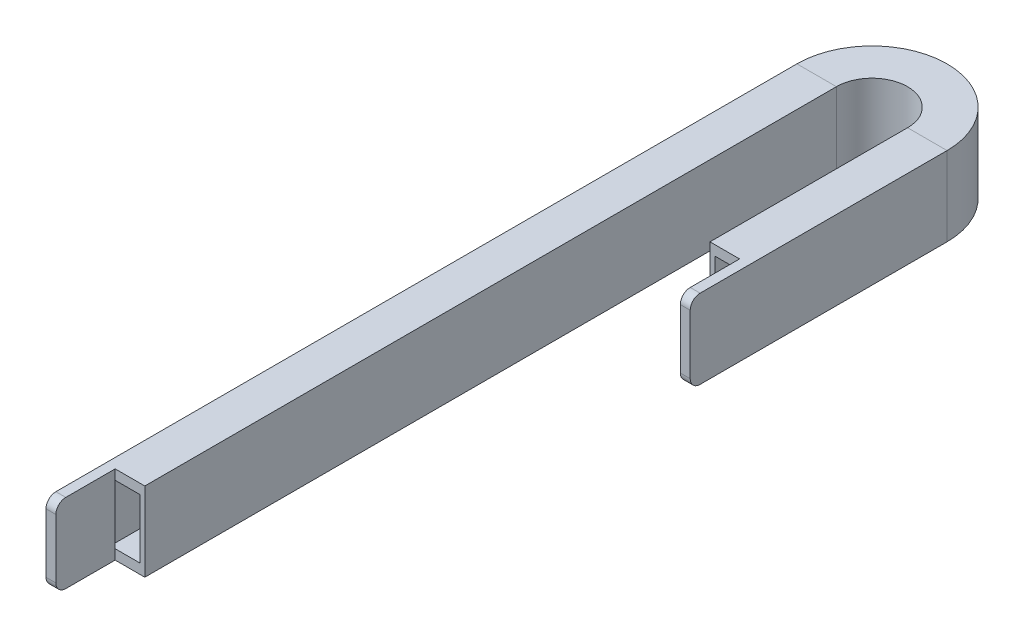
from build123d import *

# Parameters (mm, degrees)
SKETCH_1_W      = 20
SKETCH_1_H      = 40
SKETCH_11_W     = 15
SKETCH_11_H     = 30
SKETCH_3_W      = 5
SKETCH_3_H      = 40
EXTRUDE_1_DEPTH = 30
FILLET_1_R      = 5
SKETCH_5_W      = 5
SKETCH_5_H      = 40
EXTRUDE_2_DEPTH = 30
FILLET_2_R      = 5


with BuildPart() as part:
    # Sweep 1: sweep along a path in 草图2
    with BuildLine(Plane(origin=(0, 0, 0), x_dir=(1, 0, 0), z_dir=(0, 1, 0))) as sweep_1_path:
        Line((0, 0), (0, 350))
        ThreePointArc((0, 350), (28, 378), (56, 350))
        Line((56, 350), (56, 250))
    # 草图1 → Sweep 1 (sweep)
    with BuildSketch(Plane.XY):
        Rectangle(SKETCH_1_W, SKETCH_1_H)
    sweep(path=sweep_1_path.line)

    # Sweep 1 2: sweep along a path in 草图12
    with BuildLine(Plane(origin=(0, 0, 0), x_dir=(1, 0, 0), z_dir=(0, 1, 0))) as sweep_1_2_path:
        Line((0, 0), (0, 350))
        ThreePointArc((0, 350), (28, 378), (56, 350))
        Line((56, 350), (56, 243.98141307))
    # 草图11 → Sweep 1 2 (sweep, cut)
    with BuildSketch(Plane.XY):
        Rectangle(SKETCH_11_W, SKETCH_11_H)
    sweep(path=sweep_1_2_path.line, mode=Mode.SUBTRACT)

    # 草图3 → 凸台-拉伸1 (add)
    with BuildSketch(Plane.XY):
        with Locations((-7.5, 0)):
            Rectangle(SKETCH_3_W, SKETCH_3_H)
    extrude(amount=EXTRUDE_1_DEPTH)

    # 圆角1
    fillet_1_edges = [part.edges().sort_by_distance(p)[0] for p in [
        (-7.5, 20, 30),
        (-7.5, -20, 30),
    ]]
    fillet(fillet_1_edges, radius=FILLET_1_R)

    # 草图5 → 凸台-拉伸2 (add)
    with BuildSketch(Plane.XY.offset(-250)):
        with Locations((63.5, 0)):
            Rectangle(SKETCH_5_W, SKETCH_5_H)
    extrude(amount=EXTRUDE_2_DEPTH)

    # 圆角2
    fillet_2_edges = [part.edges().sort_by_distance(p)[0] for p in [
        (63.5, 20, -220),
        (63.5, -20, -220),
    ]]
    fillet(fillet_2_edges, radius=FILLET_2_R)


solid = part.part
